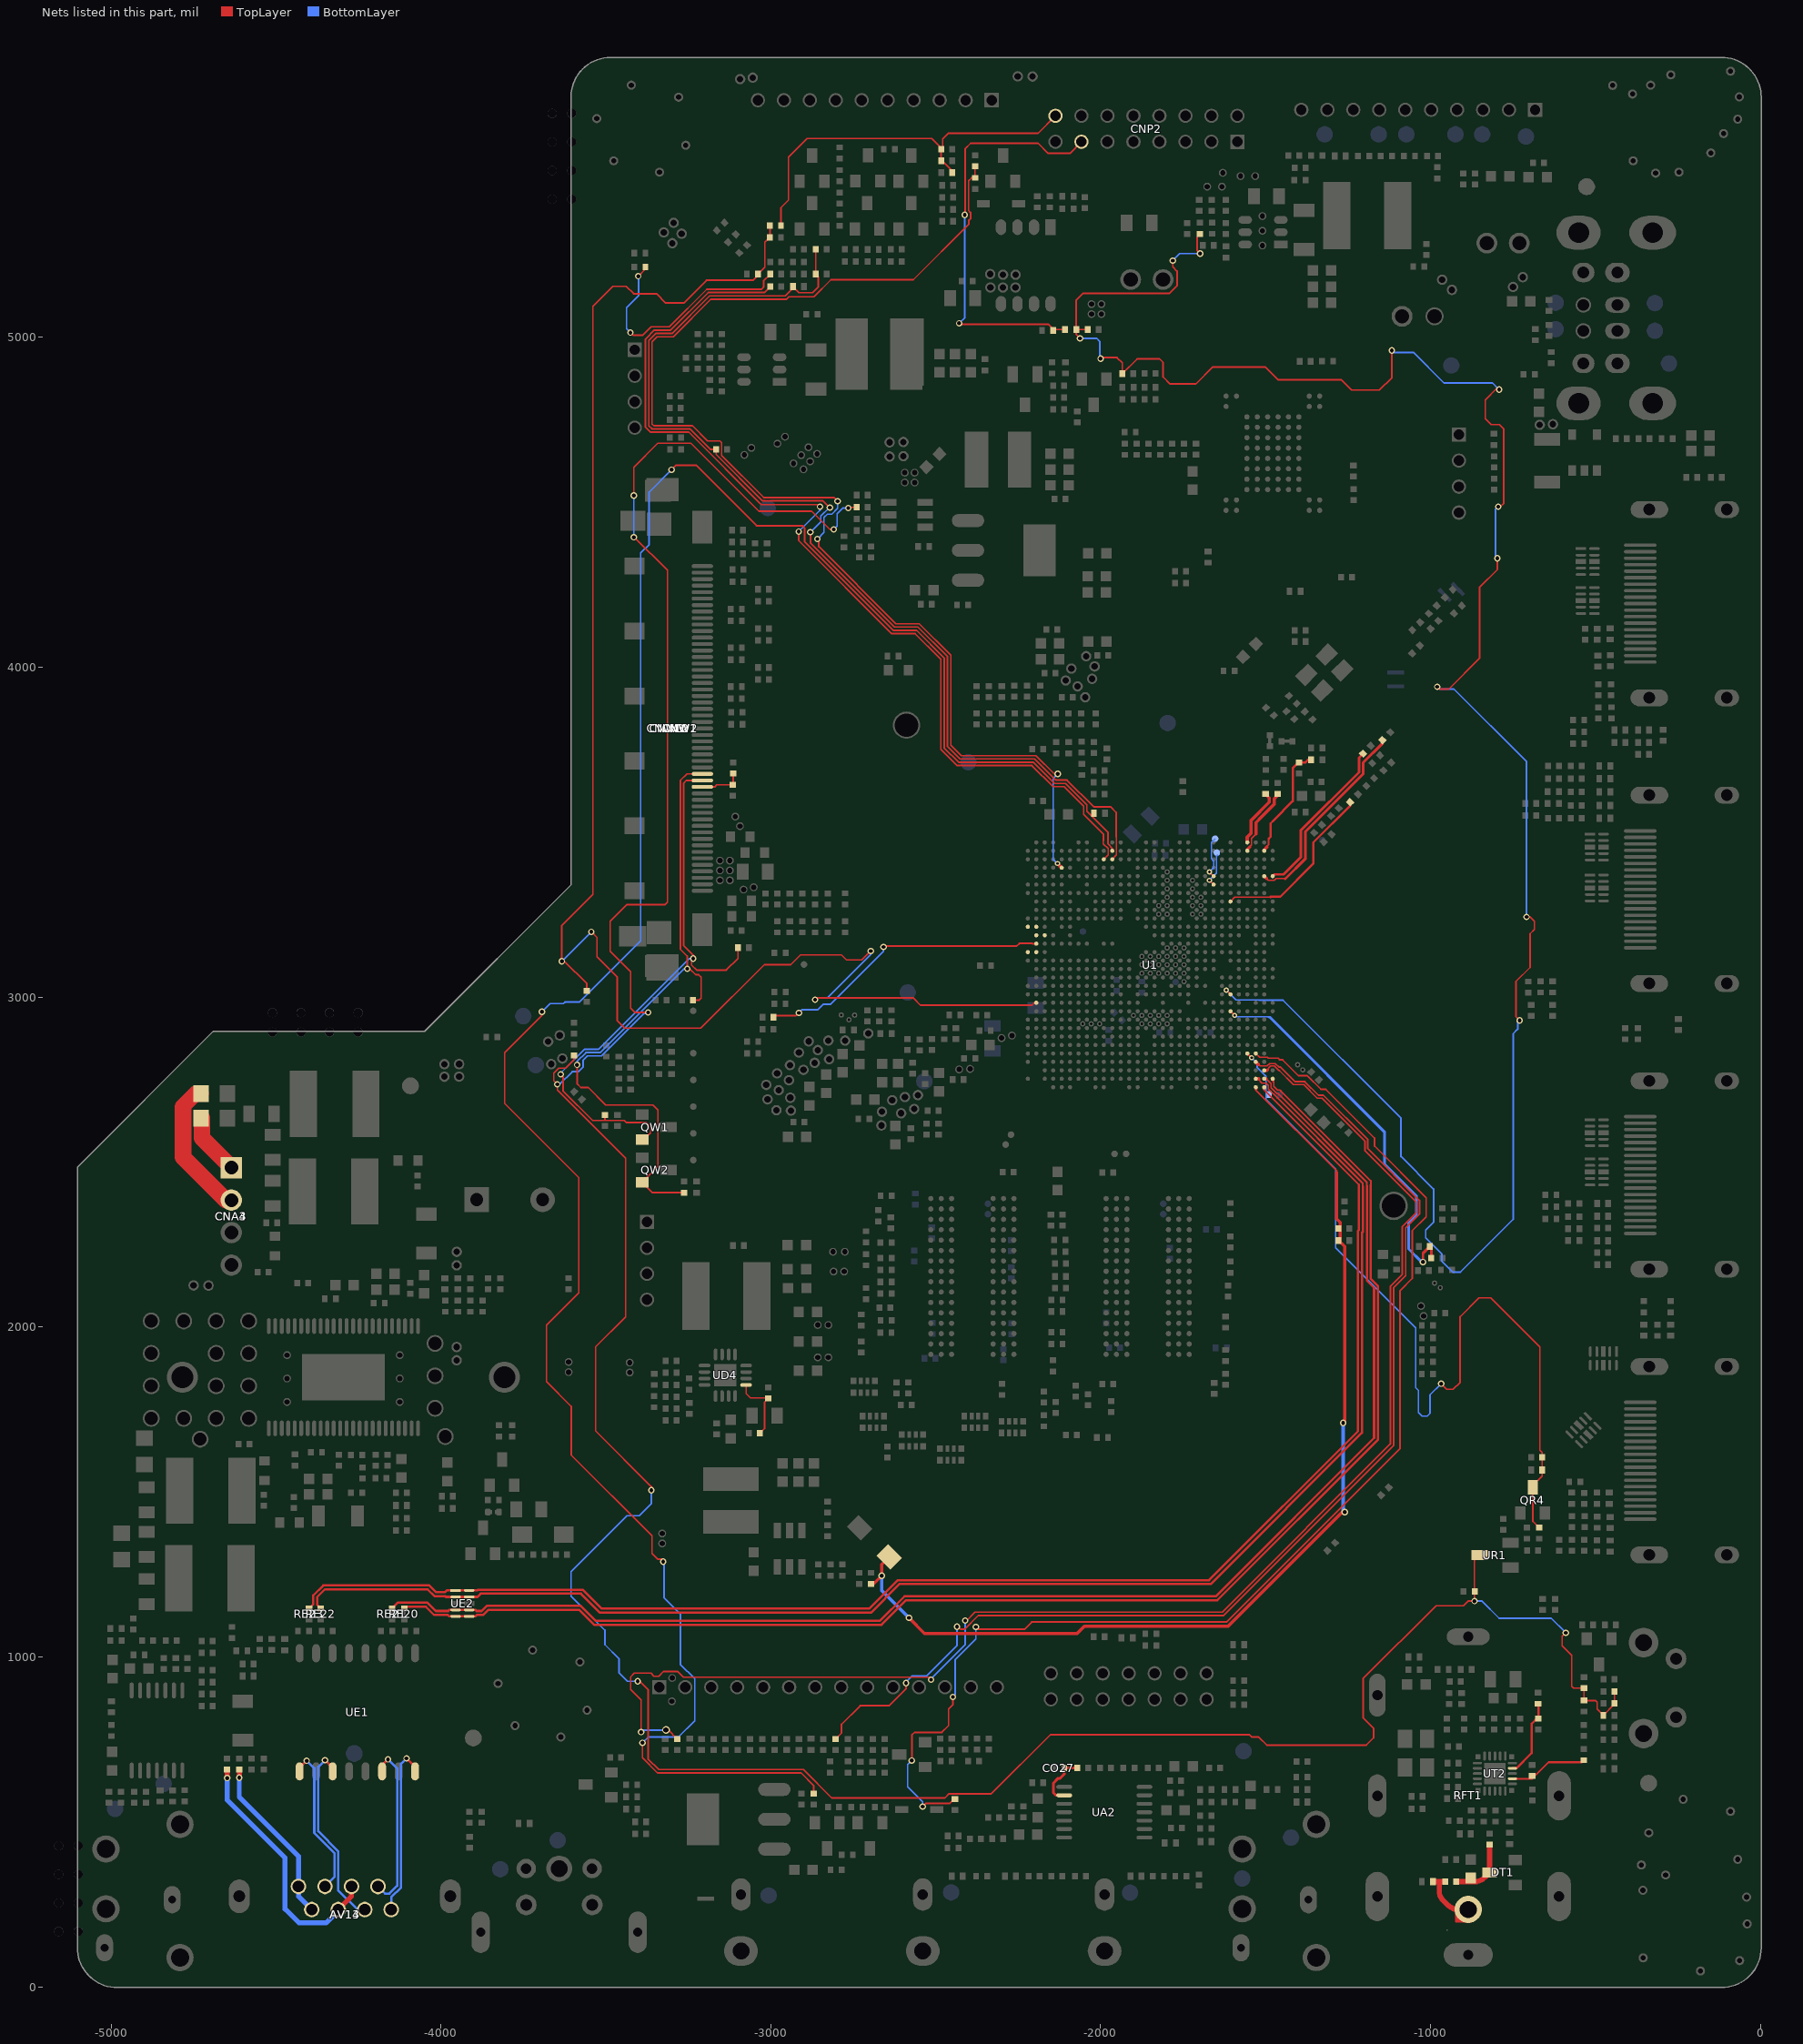
[diagram p0: the nets of this part, all layers, seen from the top]
# Altium PCB MISC86290.PcbDoc (part 27 of 31)
Units mil, origin at the board's own origin, x right, y up, seen from the top; angles counter-clockwise.
Board outline 5104.71 x 5851.49 mil, 2 copper layers (TopLayer, BottomLayer), stack 61.855 mil thick; 1026 components, 667 nets, 4280 pads, 2294 vias.

## Via types
v1: diameter 19.68, hole 11.81, TopLayer to BottomLayer, tented both sides, 1189 vias
v2: diameter 19.68/19.68 (per signal layer), hole 11.81, TopLayer to BottomLayer, tented both sides, 366 vias
v3: diameter 15.75, hole 7.87, TopLayer to BottomLayer, tented both sides, 348 vias
v4: diameter 23.62, hole 15.75, TopLayer to BottomLayer, tented both sides, 309 vias
v5: diameter 15.75/15.75 (per signal layer), hole 7.87, TopLayer to BottomLayer, tented both sides, 59 vias
v6: diameter 24/24 (per signal layer), hole 16, TopLayer to BottomLayer, tented both sides, 23 vias

## Nets (pads, with @x,y where several pads share a name; then routed paths per layer and width w, separated by ;. In a path a pad name is that pad's centre, name@x,y a point inside that pad or via, vN(x,y) a via of type N, cw(c..) or ccw(c..) an arc to the next point about the centre after c; other vN are vias at no path point) (continued)
PCID_EN: CNW1.35 CNW2.35 CNW3.35 CNW12.35 RW408.1 RW415.2 | length 128.8
  TopLayer w5: CNW3.35@-3207.67,3637.36 -3170.25,3637.36 -3163.88,3643.73 RW408.1@-3115,3643.73 ; RW408.1@-3114,3644.73 RW415.2@-3114,3678.27
PHY_RX_N: RE23.1 U1.A2 UE2.1 UE2.8 | length 4645.8
  TopLayer w6: U1.A2@-1504.25,2726.97 -1504.25,2718.76 -1217.25,2431.76 -1217.25,2429.72
  TopLayer w7: RE23.1@-4400,1146.75 -4387.5,1159.29 -4387.5,1186 -4357,1216.5 -4035.29,1216.5 -4014.79,1196 -3988,1196 -3982.63,1201.37 UE2.1@-3955.47,1201.37 UE2.8@-3914.53,1201.37 -3890.32,1201.37 -3888.04,1203.66 -3570.44,1203.66 -3512.78,1146 -2701.84,1146 -2615.23,1232.61 -2531.78,1232.61 -2516.45,1232.61 -1671.49,1232.61 -1220.22,1683.87 -1220.22,2290.75 -1217.25,2293.72 -1217.25,2429.72
PHY_RX_P: RE22.1 U1.B3 UE2.2 UE2.7 | length 4703.5
  TopLayer w3.94: U1.B3@-1523.94,2752.56 -1510.51,2739.14 -1498.14,2739.14 -1491.46,2732.46 -1491.46,2721.56 -1464.69,2694.79
  TopLayer w6: -1464.69,2694.79 -1220.89,2451 ; -1220.89,2450.96 -1205.75,2435.81 -1205.75,2425.5 -1205.25,2426
  TopLayer w7: RE22.1@-4364.5,1146.75 -4375.5,1157.79 -4375.5,1181.03 -4352.03,1204.5 -4040.26,1204.5 -4019.76,1184 -3987,1184 -3984.69,1181.69 UE2.2@-3955.47,1181.69 UE2.7@-3914.53,1181.69 -3889.32,1181.69 -3879.34,1191.66 -3575.41,1191.66 -3517.75,1134 -2696.87,1134 -2610.26,1220.61 -2536.75,1220.61 -2511.48,1220.61 -1666.52,1220.61 -1208.22,1678.9 -1208.22,2285.78 -1205.25,2288.75 -1205.25,2426
  TopLayer w10: U1.B3@-1529.84,2752.56 -1523.94,2752.56 -1520.79,2752.56 -1520.55,2752.32
PHY_TX_N: RE21.1 U1.B2 UE2.3 UE2.6 | length 4484.3
  TopLayer w3.94: U1.B2@-1498.56,2752.56 -1483.58,2737.58 -1483.58,2725.49 -1465.72,2707.63 -1461.92,2707.63 -1458.65,2704.36
  TopLayer w6: -1458.65,2704.36 -1193.25,2438.96 -1193.25,2427
  TopLayer w7: RE21.1@-4148.5,1146.75 -4131.18,1164.11 -4040.88,1164.11 -4015.77,1139 -3978.31,1139 -3974.99,1142.32 UE2.3@-3955.47,1142.32 UE2.6@-3914.53,1142.32 -3895.32,1142.32 -3892,1139 -3876.84,1139 -3861.18,1154.66 -3576.6,1154.66 -3530.94,1109 -2669.54,1109 -2594.93,1183.61 -2552.07,1183.61 -2496.15,1183.61 -1651.19,1183.61 -1171.22,1663.58 -1171.22,2118.65 -1193.25,2140.68 -1193.25,2427
  TopLayer w10: U1.B2@-1504.25,2752.56 U1.B2@-1499.5,2752.5
PHY_TX_P: RE20.1 U1.B1 UE2.4 UE2.5 | length 4457.1
  TopLayer w3.94: U1.B1@-1478.66,2746.58 -1478.66,2745.3 -1477.26,2743.9 ; -1475.71,2743.9 -1475.71,2729.52 -1464.42,2718.23 -1456.92,2718.23 -1454.62,2715.93
  TopLayer w6: -1454.62,2715.93 -1181.25,2442.56 -1181.25,2430
  TopLayer w7: RE20.1@-4111.5,1146.75 -4106.25,1152 -4045.74,1152 -4020.74,1127 -3979.31,1127 -3974.94,1122.63 UE2.4@-3955.47,1122.63 UE2.5@-3914.53,1122.63 -3896.06,1122.63 -3891.69,1127 -3871.87,1127 -3856.21,1142.66 -3581.57,1142.66 -3535.91,1097 -2664.57,1097 -2589.96,1171.61 -2557.04,1171.61 -2491.18,1171.61 -1646.22,1171.61 -1159.22,1658.61 -1159.22,2123.62 -1181.25,2145.65 -1181.25,2430
  TopLayer w8: U1.B1@-1478.66,2752.56 -1478.66,2748.18 U1.B1@-1477.07,2746.58
PIN4&5: AV13.4 AV13.5 AV14.4 AV14.5 RE4.2 | length 780
  TopLayer w15: RE4.2@-4648.5,658.5 -4648.5,633 v1(-4648,632.5) ; AV13.5@-4311.47,233.86 -4271.31,274.02 AV13.4@-4271.31,303.94
  BottomLayer w15: v1(-4648,632.5) -4648,566 -4472.5,390.5 -4472.5,235.5 -4430.17,193.17 -4348.83,193.17 -4311.47,230.53 AV13.5@-4311.47,233.86
PIN7&8: AV13.7 AV13.8 AV14.7 AV14.8 RE3.2 | length 515.7
  TopLayer w15: v1(-4611.5,633.5) -4611.33,633.67 RE3.2@-4611.33,658.5
  BottomLayer w15: v1(-4611.5,633.5) -4611.5,575 -4431.94,395.44 AV13.8@-4431.94,303.94 -4431.94,274.02 AV13.7@-4391.78,233.86
PM_RX_IC: PM_RX.1 U1.AE8 | length 106.5
  TopLayer w3.94: v3(-1670.59,3353.94) U1.AE8@-1657.8,3341.14
  BottomLayer w3.94: v3(-1670.59,3353.94) -1648.9,3375.63 -1648.9,3427.79 PM_RX.1@-1645,3431.69
PM_TX_IC: PM_TX.1 U1.AF8 | length 132.2
  TopLayer w3.94: v3(-1670.59,3379.53) U1.AF8@-1657.8,3366.73
  BottomLayer w3.94: v3(-1670.59,3379.53) -1656.85,3393.27 -1656.85,3412.37 -1664.5,3420.02 -1664.5,3468.5 PM_TX.1@-1653,3480
PS_ON: CNP2.13 RP5.1 RP8.1 | length 1249
  TopLayer w5: v1@-2426.25,5040 -2159,5040 -2144.27,5025.27 -2144.27,5024 RP8.1@-2107.73,5024 ; v1(-2412,5371.5) -2410.43,5373.07 -2410.43,5572.28 -2394.22,5588.5 -2189.75,5588.5 -2159.25,5558 -2093.21,5558 CNP2.13@-2058.21,5593
  BottomLayer w5: v1(-2429.25,5043) -2412,5060.25 v1(-2412,5371.5)
PWM/ADJ: CG11.2 CNP2.16 RG13.2 RG14.2 RG15.1 | length 1190.8
  TopLayer w5: RG15.1@-2969.27,5339.5 -2969.27,5393.23 -2946.34,5416.16 -2946.34,5546.03 -2889.52,5602.85 -2512.35,5602.85 -2483.73,5574.23 CG11.2@-2483.73,5570.5 -2483.73,5538.46 RG13.2@-2450.27,5505 ; CG11.2@-2479,5579 -2479,5601.5 -2462,5618.5 -2190.19,5618.5 CNP2.16@-2136.95,5671.74
PWR_EN_3: CD30.2 RD30.2 UD4.13 | length 215.1
  TopLayer w5: UD4.13@-3075.02,1824.16 -3075.02,1798.02 -3061.77,1784.77 CD30.2@-3008,1784.77 ; RD30.2@-3033.27,1678 -3019,1692.27 -3019,1772.27 CD30.2@-3007.5,1783.77
R_OUT+: CNA3.1 CNA4.1 RA32.2 | length 187
  TopLayer w50: RA32.2@-4725,2633 -4725,2632.59 -4725,2572.54 CNA4.1@-4635.54,2483.08
R_OUT-: CNA3.2 CNA4.2 RA33.2 | length 422.8
  TopLayer w47.24: -4782,2669.48 -4743.89,2707.59 RA33.2@-4727,2707.59
  TopLayer w50: -4782,2666.52 -4782,2515 -4651.66,2384.66 CNA4.2@-4635.54,2384.66
RCA_AU_LIN: CI4.2 U1.AF2 | length 613.9
  TopLayer w3.94: -1497.61,3360.09 -1491.46,3353.94 -1473.82,3353.94 -1467.91,3359.84 -1462.02,3359.84 -1457.99,3359.84
  TopLayer w5: -1457.99,3359.84 -1441.27,3359.84
  TopLayer w8: -1441.27,3359.12 -1439.92,3359.12 -1380,3419.04 -1380,3500.61 -1204,3676.62 -1204,3711 -1145.83,3769.17 CI4.2@-1145.83,3779.17
  TopLayer w10: U1.AF2@-1504.25,3366.73 -1497.61,3360.09
RCA_AU_RIN: CI6.2 U1.AF1 | length 501.2
  TopLayer w8: U1.AF1@-1478.66,3366.73 -1473.28,3372.12 -1445.3,3372.12 -1393,3424.42 -1393,3506 -1217,3682 -1217,3726 CI6.2@-1204.83,3738.17
RCA_CVBSIN: CI2.2 U1.AC6 | length 530.8
  TopLayer w3.94: U1.AC6@-1606.61,3289.96 -1593.96,3302.61 -1485.19,3302.61
  TopLayer w7: -1485.19,3303.8 -1484.63,3304.37 -1455.94,3304.37 -1355.5,3404.8 -1355.5,3468.5 -1243.83,3580.17 CI2.2@-1243.83,3591.17
RF_IN: CT25.1 LT4.1 NC/ESD.2 RFT1.1 | length 169.7
  TopLayer w15.8: LT4.1@-992.96,318.3 CT25.1@-955.43,318.3 ; -973.7,317.3 -973.7,290.09 ccw(c-932.91,290.09) -961.77,261.27 -951.07,250.57 ccw(c-899,302.63) -924.33,233.49 ccw(c-899,302.63) -923.47,233.18 ccw(c-899,302.63) -921.73,232.6 ccw(c-899,302.63) -907.55,229.5 ccw(c-899,302.63) -899.72,229 ccw(c-899,302.63) RFT1.1@-899,229
RF_INPUT: CT25.2 DT1.2 LT9.1 RT3.1 | length 195.2
  TopLayer w15.8: CT25.2@-921.96,318.3 -867.16,318.3 ccw(c-867.16,362.76) -835.72,331.32 DT1.2@-820.89,346.15 RT3.1@-820.89,430.63
RINN: CO27.2 RO55.2 UA2.2 | length 168
  TopLayer w8: UA2.2@-2110.55,580.18 -2135.8,580.18 -2143.67,588.05 -2143.67,617.33 -2129,632 -2123,632 -2110.26,644.74 CO27.2@-2110.26,663 RO55.2@-2070.96,663
RJ45_FE_RX+: AV13.3 AV14.3 UE1.11 | length 575.6
  TopLayer w7: v1(-4351.5,686.5) -4328.5,663.5 UE1.11@-4328.5,652.87
  BottomLayer w7: v1(-4351.5,686.5) -4372,666 -4372,471 -4311,410 -4311,291.5 -4253.36,233.86 AV13.3@-4231.15,233.86
RJ45_FE_RX-: AV13.6 AV14.6 UE1.9 | length 468.8
  TopLayer w7: UE1.9@-4428.5,652.87 -4428.5,663.5 v1(-4407,685)
  BottomLayer w7: v1(-4407,685) -4384,662 -4384,466.03 -4323,405.03 -4323,332.56 AV13.6@-4351.62,303.94
RJ45_FE_TX+: AV13.1 AV14.1 UE1.16 | length 537.6
  TopLayer w7: v1(-4104.5,692.5) -4078.5,666.5 UE1.16@-4078.5,652.87 UE1.16@-4078.5,643.5
  BottomLayer w7: AV13.1@-4150.84,233.86 -4150.84,271.19 -4121,301.03 -4121,676 v1(-4104.5,692.5)
RJ45_FE_TX-: AV13.2 AV14.2 UE1.14 | length 514.6
  TopLayer w7: UE1.14@-4178.5,652.87 -4178.5,671 v1(-4160.5,689)
  BottomLayer w7: AV13.2@-4190.99,303.94 -4169.54,282.49 -4156.51,282.49 -4133,306 -4133,661.5 v1(-4160.5,689)
RST_BTNN: RR11.1 U1.E3 | length 3827
  TopLayer w3.94: U1.E3@-1529.84,2829.33 -1517.67,2817.16 -1495.04,2817.16 -1492.44,2814.57 -1461.93,2814.57 -1457.21,2809.85 -1456.35,2809.85
  TopLayer w5: v1(-2573.04,685.73) -2572.31,685 -2572.31,762.69 -2564,771 -2481.52,771 -2461,791.52 -2461,841.64 -2448.34,854.3 v1(-2448.34,878.61) ; v1(-2539.85,546.18) -2530.54,555.5 -2458,555.5 -2444.77,568.73 RR11.1@-2442,568.73 ; v1(-2378.5,1091) -2371,1083.5 -2231.5,1083.5 -2209.39,1105.61 -1618.88,1105.61 -1092.22,1632.27 -1092.22,2110.35 -1055.5,2147.07 -1055.5,2292.18 -1013.5,2334.18 -1013.5,2392.04 -1169.9,2548.44 -1169.9,2572.61 -1317.78,2720.48 -1332.46,2720.48 -1373.57,2761.6 -1400.18,2761.6 -1448.43,2809.85 -1456.35,2809.85
  BottomLayer w5: v1(-2573.04,685.73) -2585.37,673.39 -2585.37,606.21 -2539.85,560.69 v1(-2539.85,546.18) ; v1(-2448.34,878.61) -2441,885.95 -2441,991.86 -2378.5,1054.36 v1(-2378.5,1091)
RST_BTNN_LATCH: DR5.K RR14.2 U1.AJ20 | length 7226.3
  TopLayer w3.94: -1977.76,3464.39 -1977.76,3463.76 -1964.88,3450.89 U1.AJ20@-1964.88,3443.5
  TopLayer w5: v1(-3694,2955.5) -3694,2944.08 -3806.9,2831.18 -3806.9,2677.88 -3582.15,2453.12 -3582.15,2103.03 -3679.9,2005.28 -3679.9,1834.22 -3604.9,1759.22 -3604.9,1611.79 -3360.34,1367.23 -3360.34,1313.03 -3343.71,1296.41 v1@-3326.41,1296.41 ; v1(-3389,739.5) -3389,693.75 -3343.43,648.18 -2908.15,648.18 -2870.25,610.27 RR14.2@-2870.25,585.73 ; v1(-3301,4599) -3287.34,4612.66 -3226.87,4612.66 -3043.55,4429.34 -2904.34,4429.34 -2897.84,4422.84 -2897.84,4380.88 -2628.96,4112 -2558.43,4112 -2474.5,4028.07 -2474.5,3755.53 -2431.08,3712.11 -2204.17,3712.11 -2140.06,3648 -2106.46,3648 -2041.9,3583.44 -2041.9,3563.4 -1978.29,3499.79 -1978.29,3464.39
  BottomLayer w5: v1(-3694,2955.5) -3669.16,2980.34 -3628.72,2980.34 -3624.05,2985.01 -3580.89,2985.01 -3394.61,3171.29 -3394.61,4346.58 -3369,4372.2 -3369,4531 v1(-3301,4599) ; v1(-3389,739.5) -3371.5,757 -3280.14,757 -3230.73,806.41 -3230.73,933.94 -3274.25,977.46 -3274.25,1130.11 -3324.07,1179.93 v1@-3324.07,1286.26
  other v1: -3326.41,1288.6
SAR0: RK26.1 U1.D3 | length 3592.2
  TopLayer w3.94: -1522.6,2796.5 -1517.05,2790.94 -1495.65,2790.94 -1487.81,2798.78 -1470.67,2798.78 ; -1470.71,2798.82 -1470.67,2798.78 ; -1459,2787.11 -1470.67,2798.78
  TopLayer w5: RK26.1@-2803.64,751 -2786,768.64 -2786,795.25 -2729.25,852 -2641.5,852 -2590,903.5 v1(-2590,920.5) ; v1(-2435.5,1091.5) -2432.5,1091.5 -2424.5,1083.5 -2412.91,1083.5 -2370.8,1125.61 -1627.17,1125.61 -1112.22,1640.55 -1112.22,2118.63 -1075.5,2155.36 -1075.5,2300.46 -1033.5,2342.46 -1033.5,2383.75 -1190.32,2540.57 -1190.32,2567.85 -1325.15,2702.68 -1339.83,2702.68 -1380.94,2743.8 -1410.66,2743.8 -1454.67,2787.81 -1458.3,2787.81
  TopLayer w10: U1.D3@-1529.84,2803.74 -1522.6,2796.5
  BottomLayer w5: v1@-2590,924 -2572.5,941.5 -2528.5,941.5 -2435.5,1034.5 v1(-2435.5,1091.5)
SAR1: RK33.1 U1.C2 | length 4394.7
  TopLayer w3.94: -1497.36,2778.15 -1484.57,2790.94 -1473.92,2790.94 -1460.08,2777.11
  TopLayer w5: v1(-3393.2,771.8) -3393.2,869.39 -3425,901.19 -3425,939 -3413.5,950.5 -3363.53,950.5 -3354.18,941.16 -3339.82,941.16 -3324.97,956 -3283.14,956 -3265.46,938.31 -2518.31,938.31 -2514,934 v1(-2514,930.5) ; v4(-3318,778) -3311.06,778 RK33.1@-3284.06,751 ; v1(-2411,1110) -2406.24,1110 -2380.63,1135.61 -1631.31,1135.61 -1121.72,1645.2 -1121.72,2123.28 -1085.5,2159.5 -1085.5,2304.6 -1043.5,2346.6 -1043.5,2379.61 -1199.22,2535.33 -1199.22,2564.17 -1328.84,2693.78 -1343.51,2693.78 -1384.63,2734.9 -1415.91,2734.9 -1458.12,2777.11
  TopLayer w10: U1.C2@-1504.25,2778.15 -1497.36,2778.15 -1495.79,2778.15 -1494.96,2778.98
  BottomLayer w5: v1(-3393.2,771.8) -3387,778 v4(-3318,778) ; v1(-2514,930.5) v1@-2512.34,932.16 ; v1@-2514,933.81 -2411,1036.81 v1(-2411,1110)
SAR5_VDET: C174.2 DD2.K R121.1 R123.2 U1.A3 | length 3170
  TopLayer w3.94: U1.A3@-1529.84,2723.38 -1529.84,2719.09 -1283.72,2472.98
  TopLayer w10: R121.1@-2696.16,1221.27 -2688.73,1221.27 v1(-2664,1246) -2664,1279.92 DD2.K@-2641.46,1302.46 ; v1(-2581,1118) -2534,1071 -2071.5,1071 -2049.39,1093.11 -1613.71,1093.11 -1267.82,1439 v1(-1260,1439) ; U1.A3@-1529.84,2726.97 -1529.02,2726.14 U1.A3@-1529.02,2723.38 ; -1284.7,2468.84 -1284.7,2328.5 -1273.73,2317.53 C174.2@-1273.73,2257.73 ; C174.2@-1278,2262 C174.2@-1273.73,2257.73 ; v1(-1265,1709) -1260.02,1713.98 -1260.02,2244.02 C174.2@-1273.73,2257.73
  BottomLayer w10: v1(-2664,1246) -2664,1201 v1(-2581,1118) ; v1(-1265,1709) -1265,1444 v1(-1260,1439)
SCL_VB1_OUT: CNW1.33 CNW2.33 CNW3.33 CNW12.33 QW2.S RW395.1 RW421.1 | length 1965.8
  TopLayer w5: v1(-3587.34,2794.66) -3587.34,2737.34 -3576,2726 -3553.5,2726 -3500.41,2672.91 -3357.86,2672.91 -3342.5,2657.56 -3342.5,2486.5 -3390,2439 QW2.S@-3390,2438.5 QW2.S@-3387.75,2436.25 ; QW2.S@-3390,2434 -3386,2434 -3359.27,2407.27 RW395.1@-3263,2407.27 ; v1(-3253.34,3085.81) -3253.34,3124.34 -3274,3145 -3274,3657.25 -3254.52,3676.73 CNW3.33@-3207.67,3676.73 ; v1@-3245.81,3085.81 -3228,3068 -3219,3068 -3211.5,3060.5 -3211.5,2996.5 -3217,2991 RW421.1@-3235.77,2991
  BottomLayer w5: v1(-3587.34,2794.66) -3587.34,2805.35 -3560.68,2832.01 -3517.52,2832.01 -3263.72,3085.81 v1(-3253.34,3085.81)
SDA_VB1_OUT: CNW1.34 CNW2.34 CNW3.34 CNW12.34 QW1.S RW73.1 RW393.1 | length 1795.1
  TopLayer w5: -3629.91,2758.7 -3629.91,2715.7 -3540.21,2626 -3503,2626 ; RW393.1@-3503,2642.73 -3503,2626 ; QW1.S@-3391,2568.5 QW1.S@-3390,2568.5 -3384.5,2568.5 -3364.5,2588.5 -3364.5,2607.19 -3377.56,2620.25 -3438.25,2620.25 -3444,2626 -3503,2626 ; v1@-3240,3117 -3240,3097 -3225,3082 -3135,3082 -3099.73,3117.27 RW73.1@-3099.73,3150 ; v1(-3235.5,3117) -3230.63,3121.87 -3230.63,3122.63 -3264,3156 -3264,3649.25 -3256.2,3657.05 CNW3.34@-3207.67,3657.05
  BottomLayer w5: v1(-3637.09,2765.88) -3638,2766.79 -3638,2768.83 -3564.82,2842.01 -3521.66,2842.01 -3246.67,3117 v1(-3235.5,3117)
SOC_BL_ADIM: R130.2 RG33.1 | length 743.8
  TopLayer w5: v1(-3425.5,5014.5) -3418,5007 -3387.97,5007 -3377.66,5017.32 ; v1(-3401.84,5185.46) -3380.27,5207.04 R130.2@-3380.27,5214 ; -3377.66,5017.34 -3362.9,5032.1 -3308.04,5032.1 -3194.14,5146 -3028,5146 -3022,5152 -3022,5171 -3001.73,5191.27 RG33.1@-3001.73,5192
  BottomLayer w5: v1(-3425.5,5014.5) -3437.34,5026.34 -3437.34,5089.66 -3401,5126 -3401,5184.62 v1(-3401.84,5185.46)
SOC_BL_ON: DG1.K RG2.2 RG5.2 RG6.1 U1.AH20 | length 3337
  TopLayer w3.94: U1.AH20@-1964.88,3417.91 -1952.09,3430.71 -1952.09,3484.9
  TopLayer w5: v1@-2880,4409 -2880,4377.18 -2624.82,4122 -2554.28,4122 -2464.5,4032.22 -2464.5,3759.67 -2426.94,3722.11 -2200.03,3722.11 -2135.92,3658 -2102.32,3658 -2021.32,3577 -1970,3577 -1953,3560 -1953,3485.81 ; RG2.2@-2863.73,5267 RG5.2@-2863.73,5192 -2856.5,5184.77 -2856.5,5152.5 -2873.33,5135.67 -2914.4,5135.67 DG1.K@-2932.73,5154 -2932.73,5149.27 -2956,5126 -3185.86,5126 -3299.76,5012.1 -3348.86,5012.1 -3370,4990.96 -3370,4732.14 -3360.7,4722.84 -3245.21,4722.84 -3183.36,4661 RG6.1@-3165.96,4661 -3165.96,4645.46 -3025.16,4504.66 -2841.91,4504.66 v1(-2821.25,4484)
  BottomLayer w5: v1(-2880.5,4409.5) -2848.83,4441.17 -2848.83,4458.31 v1@-2823.14,4484
SOC_BL_PDIM: DG11.K RG11.2 RG15.2 RG16.1 U1.L29 | length 5110.6
  TopLayer w5: v1(-3633.51,3108.63) -3633.51,3217.53 -3539.61,3311.42 -3539.61,5094.49 -3479.1,5155 -3438.33,5155 -3415.67,5132.34 -3346.2,5132.34 -3318.36,5104.5 -3263.93,5104.5 -3195.08,5173.34 -3053.87,5173.34 -3039.27,5187.94 DG11.K@-3039.27,5192 -3018.09,5213.18 -3018.09,5288.14 RG11.2@-3002.73,5303.5 RG15.2@-3002.73,5339.5 ; v1@-3625.78,3108.63 -3557.76,3040.6 RG16.1@-3557.76,3018.93 ; v1(-3544,3198) -3527.13,3181.13 -3527.13,3122.28 -3465.34,3060.49 -3465.34,2927.92 -3443.43,2906 -3212.08,2906 -3019.74,3098.34 -2939.59,3098.34 -2909.94,3128 -2786,3128 -2770.66,3112.66 -2724.34,3112.66 v1(-2697,3140) ; v1@-2860,2998 -2569.23,2998 -2546.76,2975.53 ; -2545.51,2975.53 -2208.22,2975.53 -2200.88,2982.87 U1.L29@-2195.2,2982.87
  BottomLayer w5: v1@-3633.37,3108.63 v1(-3544,3198) ; v1@-2860,2998 -2827.78,2998 -2697,3128.78 v1(-2697,3140)
  other v1: -2866,2992
SOC_BOOSTER: RG32.1 U1.AH21 | length 3014.2
  TopLayer w3.94: -1992,3475.11 -1992,3464.72 -1977.68,3450.39 -1977.68,3430.71 U1.AH21@-1990.47,3417.91
  TopLayer w5: RG32.1@-3001.73,5154 -3019.73,5136 -3190,5136 -3303.9,5022.1 -3353,5022.1 -3380,4995.1 -3380,4728 -3365.34,4713.34 -3249.14,4713.34 -3028.8,4493 v1@-2857.44,4493 ; v1(-2915.5,4411.5) -2915.5,4384.4 -2633.1,4102 -2562.57,4102 -2489.25,4028.68 -2484.5,4023.93 -2484.5,3751.38 -2435.23,3702.11 -2208.31,3702.11 -2144.2,3638 -2110.61,3638 -2051.9,3579.29 -2051.9,3554.53 -1992,3494.63 -1992,3475.11
  BottomLayer w5: v1(-2915.5,4411.5) -2851.13,4475.87 v1(-2851.13,4486.69)
SOC_PANEL_ON: RM11.1 RM12.2 U1.AG26 | length 3879.4
  TopLayer w5: v1(-2858.84,4388.78) -2854.5,4384.44 -2854.5,4365.82 -2620.68,4132 -2550.14,4132 -2454.5,4036.36 -2454.5,3763.81 -2422.8,3732.11 -2195.88,3732.11 -2140.63,3676.86 v1(-2130.25,3676.86) v1@-2132.77,3674.34 ; v1(-2797.64,4503.13) -2809.17,4514.66 -3021.72,4514.66 -3149,4641.93 -3149,4681 -3154,4686 -3191.5,4686 -3237.84,4732.34 -3354.84,4732.34 -3360,4737.5 -3360,4986.82 -3344.72,5002.1 -3295.61,5002.1 -3181.72,5116 -2951.86,5116 -2944.86,5123 -2869.62,5123 -2817.62,5175 -2568.06,5175 -2399.5,5343.56 -2399.5,5355.27 -2394.66,5360.11 -2394.66,5378.68 -2400.43,5384.46 -2400.43,5475.07 -2391.65,5483.85 RM11.1@-2380.81,5483.85 ; RM11.1@-2381,5484.05 RM12.2@-2381,5518.77
  TopLayer w10: v3(-2131.22,3405.12) U1.AG26@-2118.43,3392.32
  BottomLayer w3.94: -2144.26,3662.85 -2144.26,3418.15 v3(-2131.22,3405.12)
  BottomLayer w5: v1(-2858.84,4388.78) -2838.83,4408.79 -2838.83,4454.17 -2828.66,4464.34 -2814.91,4464.34 -2797.64,4481.6 v1(-2797.64,4503.13) ; -2143.72,3663.39 v1(-2130.25,3676.86)
SOC_PS_ON: RD1.1 RM1.1 RP1.1 RP8.2 U1.M6 | length 6762.2
  TopLayer w5: v1(-2062.5,4997) -2074.27,5008.77 RP8.2@-2074.27,5024 RP8.2@-2074,5024 ; RP1.1@-2039.23,5024 RP8.2@-2074,5024 ; v1(-2000.27,4935.5) -1996.77,4939 -1950.5,4939 -1934.25,4922.75 RM1.1@-1934.25,4890 -1889.25,4935 -1821.53,4935 -1811,4924.47 -1811,4880 -1789.95,4858.95 -1711.72,4858.95 -1660.18,4910.49 -1501.4,4910.49 -1462.9,4872 -1271.4,4872 -1240.02,4840.63 -1154.84,4840.63 -1117.34,4878.12 v1(-1117.34,4960.34) ; v1(-1781.5,5233) -1781.5,5214 -1768.5,5201 -1768.5,5156.5 -1791.84,5133.16 -2053.84,5133.16 -2074,5113 RP8.2@-2074,5024 ; v1(-1698.5,5254.24) -1708,5263.74 -1708,5303.25 -1699.47,5311.77 RD1.1@-1699.47,5314 RD1.1@-1697.47,5312 ; v3(-1619.41,3021.26) U1.M6@-1606.61,3008.46 ; v1(-980,3941) -973,3934 -944.37,3934 -851.5,4026.87 -851.5,4242.5 -797.66,4296.34 v1(-797.66,4330.34) ; v1(-795.05,4487.16) -787.84,4487.16 -778.66,4496.34 -778.66,4723.51 -791.15,4736 -816.28,4736 -834,4753.72 -834,4810.74 -800.74,4844 -794.15,4844 v1(-792.25,4842.11) ; v1(-730,2929.5) -730,2929.38 -741,2940.38 -741,3047.5 -698.34,3090.16 -698.34,3192.18 -685,3205.53 -685,3230 -698,3243 v1(-709,3243)
  BottomLayer w3.94: v3(-1619.41,3021.26) -1589.88,2991.73 -1520.93,2991.73
  BottomLayer w5: v1(-2062.5,4997) -2011.84,4997 -2002.84,4988 -2002.84,4942.31 -2000.27,4939.73 v1(-2000.27,4935.5) ; v1(-1781.5,5233) -1760.26,5254.24 v1(-1698.5,5254.24) ; -1519.72,2990.53 -1447.03,2990.53 -1089.5,2633 -1089.5,2516.73 -991,2418.23 -991,2317.57 -1014.99,2293.59 -1014.99,2270.08 -965.66,2220.75 -965.66,2198.88 -933.44,2166.66 -909.28,2166.66 -749.68,2326.25 -749.68,2888.79 -735.66,2902.82 -735.66,2923.84 v1(-730,2929.5) ; v1(-1117.34,4960.34) -1111.66,4954.66 -1051.94,4954.66 -959.28,4862 -812.15,4862 v1(-792.25,4842.11) ; v1(-980,3941) -973,3934 -929,3934 -709,3714 v1(-709,3243) ; v1(-797.66,4330.34) -803.34,4336.03 -803.34,4478.87 v1(-795.05,4487.16)
SOC_RESET: DR1.K DR4.K QR4.C RR17.1 RR18.2 U1.E4 | length 2613.8
  TopLayer w3.94: U1.E4@-1555.43,2829.33 v3(-1542.64,2816.54)
  TopLayer w5: v1(-968,1828) -950.93,1810.93 -931.55,1810.93 -910.5,1831.97 -910.5,2031.18 -853.34,2088.34 -818.02,2088.34 -668.88,1939.2 -668.88,1626.63 -661.77,1619.52 RR17.1@-661.77,1605.5 DR1.K@-661.77,1566.5 -661.77,1548.28 QR4.C@-690.1,1519.95 ; QR4.C@-690.1,1514.03 -690.1,1410.83 RR18.2@-671,1391.73
  BottomLayer w5: v3(-1542.64,2816.54) -1525.21,2799.11 -1525.21,2786.05 -1498.71,2759.55 -1498.71,2690.26 -1287.67,2479.22 -1287.67,2239.86 -1044.96,1997.15 -1044.96,1815.96 -1036.74,1807.74 -1036.74,1740.56 -1026.18,1730.01 -1009.99,1730.01 -1001.66,1738.34 -1001.66,1794.34 v1(-968,1828)
SOC_RESETN: CR2.2 CR3.2 R150.1 RR3.1 RR5.1 RR6.1 RR7.1 RR8.2 UR1.3 | length 9595.3
  TopLayer w5: R150.1@-3597,2823.27 -3597,2809.83 -3622.33,2784.5 -3643,2784.5 -3658,2769.5 -3658,2746.75 v1(-3647.25,2736) -3647.25,2718.9 -3440.25,2511.9 -3440.25,2030.89 -3531,1940.14 -3531,1684.98 -3361,1514.98 ; v1(-3415.5,4520.5) -3415.5,4606.5 -3343,4679 -3242.3,4679 -3036.3,4473 -2876.11,4473 -2821.11,4418 v1(-2809.25,4418) ; v1@-3413.5,4394 -3313.5,4294 -3313.5,3287.95 -3321.45,3280 -3437,3280 -3487.13,3229.87 -3487.13,3138.85 -3425,3076.72 -3425,2967 -3411.34,2953.34 v1(-3371.66,2953.34) ; v1@-3397.09,926 -3372.09,901 -3372.09,690.27 -3340,658.18 -2904.01,658.18 -2901.15,658.18 -2815.32,572.34 -2472.66,572.34 -2460,585 -2331.4,585 -2152.4,764 -1548.89,764 ; v1@-2763.25,4485 RR6.1@-2740.17,4485 ; -1547.89,763 -1541.64,756.75 -1520.86,756.75 -1496.61,732.5 -1194.69,732.5 -1173,754.19 -1173,783.81 -1204.49,815.3 -1204.49,933.83 -983.47,1154.84 -900.16,1154.84 -886,1169 v1(-867,1169) -867,1293.24 UR1.3@-851.74,1308.5 ; v2(-590,1073) -601,1062 -601,1034 -572,1005 -572,911 -566.27,905.27 RR3.1@-535,905.27 CR3.2@-535,867.73 -500.23,867.73 -495,862.5 -495,841.27 RR8.2@-476.23,822.5 -442.27,856.46 RR5.1@-442.27,859.16 RR7.1@-442.27,895.16
  BottomLayer w5: v1@-3640,2736 -3602,2774 -3583.47,2774 -3569,2788.47 -3569,2809.55 -3556.54,2822.01 -3513.38,2822.01 -3385.39,2950 v1@-3375.01,2950 ; v1(-3415.5,4394) v1(-3415.5,4520.5) ; v1(-3403.5,926) -3434.75,926 -3460.5,951.75 -3460.5,994.5 -3503,1037 -3503,1080.86 -3605.5,1183.36 -3605.5,1258.5 -3436,1428 -3398.86,1428 -3362,1464.86 v1(-3362,1505) ; v1(-2809.25,4418) -2799.25,4428 -2799.25,4465.25 -2781.5,4483 v1(-2765.25,4483) ; v1(-867,1169) -844.14,1169 -792.14,1117 -634,1117 v2(-590,1073)
SPDIF_OUT_IC: CO3.2 RO1.1 U1.K6 | length 1180.8
  TopLayer w3.94: U1.K6@-1606.61,2957.28 v3(-1593.82,2944.49)
  TopLayer w8: v1(-1023,2197) -1023,2223.5 CO3.2@-1002.5,2244 ; RO1.1@-997.73,2208.5 CO3.2@-997.73,2239.23
  BottomLayer w3.94: v3@-1589.88,2940.55 -1496.1,2940.55 ; -1486.89,2938.36 -1489.08,2940.55 ; -1484.5,2939.1 ccw(c-1488,2935.6) -1488,2940.55 -1489.08,2940.55 ; -1496.1,2940.55 cw(c-1496.1,2930.05) -1488.68,2937.48 ccw(c-1496.1,2930.05) -1496.1,2940.55 ; -1496.1,2940.55 -1489.08,2940.55
  BottomLayer w8: -1486.33,2938.03 -1140.01,2591.71 -1140.01,2494.41 -1042.5,2396.89 -1042.5,2338.91 -1066.49,2314.92 -1066.49,2236.49 v1@-1027,2197
SPI_CLK: U1.Y30
SPI_CSN: U1.Y29
SPI_MISO: U1.W28
SPI_MOSI: U1.W29
TCON0_TX1: R202.2 U1.V29 | length 890.4
  TopLayer w5: R202.2@-2986.91,2944.12 -2922.88,2944.12 v1(-2915,2952) ; v1(-2658.5,3152) -2656,3154.5 -2255.14,3154.5 -2246.61,3163.03 -2207.67,3163.03 -2206.65,3162.01 U1.V29@-2195.2,3162.01
  BottomLayer w5: v1(-2915,2952) -2904.83,2962.17 -2857.17,2962.17 -2841.33,2978 -2819.5,2978 -2658.5,3139 v1(-2658.5,3152)
TCON2_TX2: U1.U29
TCON3_RX2: U1.U30
TUN_IF_AGC: CT10.2 RT9.1 UT2.5 | length 236
  TopLayer w7: UT2.5@-751.74,662.11 -739.95,662.11 -693.53,708.53 -693.53,797.47 -673,818 -673,855.78 RT9.1@-674.98,857.77
TUNER_AGC_IC: RT1.2 RT7.1 U1.AJ2 | length 352.2
  TopLayer w3.94: U1.AJ2@-1504.25,3443.5 U1.AJ2@-1504.11,3443.65
  TopLayer w5: -1498.17,3456.22 -1490.85,3463.54 -1490.85,3480.11
  TopLayer w7: -1490.85,3480.11 -1485,3485.96 -1485,3526.52 -1475.82,3535.7 -1475.82,3535.93 -1417.5,3594.24 -1417.5,3694.5 -1400.27,3711.73 RT7.1@-1398.5,3711.73 -1379.26,3711.73 -1371.5,3719.5 RT1.2@-1361.73,3719.5
  TopLayer w10: U1.AJ2@-1504.25,3443.5 -1504.25,3446.6 -1496.4,3454.45
TUNER_IFM_IC: CT32.2 U1.AK4 | length 175.9
  TopLayer w10: U1.AK4@-1555.43,3469.09 -1555.89,3469.55 -1555.89,3485.18 -1544.45,3496.62 -1544.45,3535.66 -1489,3591.11 -1489,3604.01 CT32.2@-1498.23,3613.24
TUNER_IFP_IC: CT27.1 U1.AJ4 | length 216.9
  TopLayer w3.94: -1548.93,3455.01 -1542.64,3461.33 -1542.64,3480.47 -1529,3494.11 -1529,3495.46
  TopLayer w9.84: -1519.45,3539.56 -1474,3585.01 -1474,3601.46 CT27.1@-1462.23,3613.24
  TopLayer w10: U1.AJ4@-1555.43,3443.5 -1555.43,3448.16 -1548.75,3454.84 ; -1529.45,3495.46 -1529.45,3529.45 -1513.39,3545.5
TUNER_SCL: CT5.1 RT8.1 UT2.3 | length 231.6
  TopLayer w6: UT2.3@-751.74,630.62 -739.17,630.62 -739.29,630.5 -692,630.5 -642.08,680.42 RT8.1@-541.08,680.42